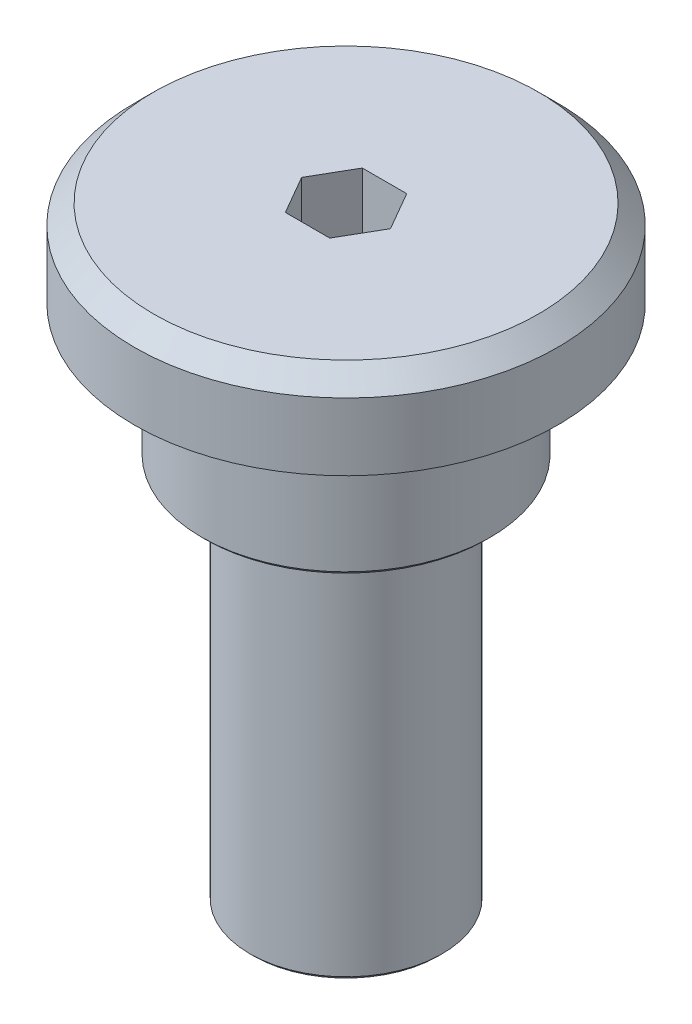
SolidWorks part; units mm, degrees
ref_plane "Front" through (0, 0, 0) normal (0, 0, 1) x (1, 0, 0)
ref_plane "Top" through (0, 0, 0) normal (0, 1, 0) x (1, 0, 0)
ref_plane "Right" through (0, 0, 0) normal (1, 0, 0) x (0, 0, -1)
sketch "草图1" plane through (0, 0, 0) normal (0, 1, 0) x (1, 0, 0)
  circle A0 centre (0, 0) radius 5
  dimension "D1" = 10
extrude "凸台-拉伸1" add sketch "草图1" along normal blind 20
cosmetic thread "装饰螺纹线1" parameters "D1"=18, "D2"=8.376
sketch "草图2" plane through (0, 20, 0) normal (0, 1, 0) x (1, 0, 0)
  circle A0 centre (0, 0) radius 7.5
  dimension "D1" = 15
extrude "凸台-拉伸2" add sketch "草图2" along normal blind 7
sketch "草图3" plane through (0, 27, 0) normal (0, 1, 0) x (1, 0, 0)
  circle A0 centre (0, 0) radius 11
  dimension "D1" = 22
extrude "凸台-拉伸3" add sketch "草图3" along normal blind 4.5
chamfer "倒角1" distance 1 angle 45 1 edges at (0, 31.5, 11)
chamfer "倒角2" distance 0.2 angle 45 1 edges at (0, 20, 7.5)
chamfer "倒角3" distance 0.2 angle 45 1 edges at (0, 0, 5)
sketch "草图4" plane through (0, 31.5, 0) normal (0, 1, 0) x (1, 0, 0)
  line L1 (2.3094, 0) -> (1.1547, 2)
  line L2 (1.1547, 2) -> (-1.1547, 2)
  line L3 (-1.1547, 2) -> (-2.3094, 0)
  line L4 (-2.3094, 0) -> (-1.1547, -2)
  line L5 (-1.1547, -2) -> (1.1547, -2)
  line L6 (1.1547, -2) -> (2.3094, 0)
  circle A0 centre (0, 0) radius 2 construction
  dimension "D1" = 4
extrude "切除-拉伸1" cut sketch "草图4" against normal blind 4
